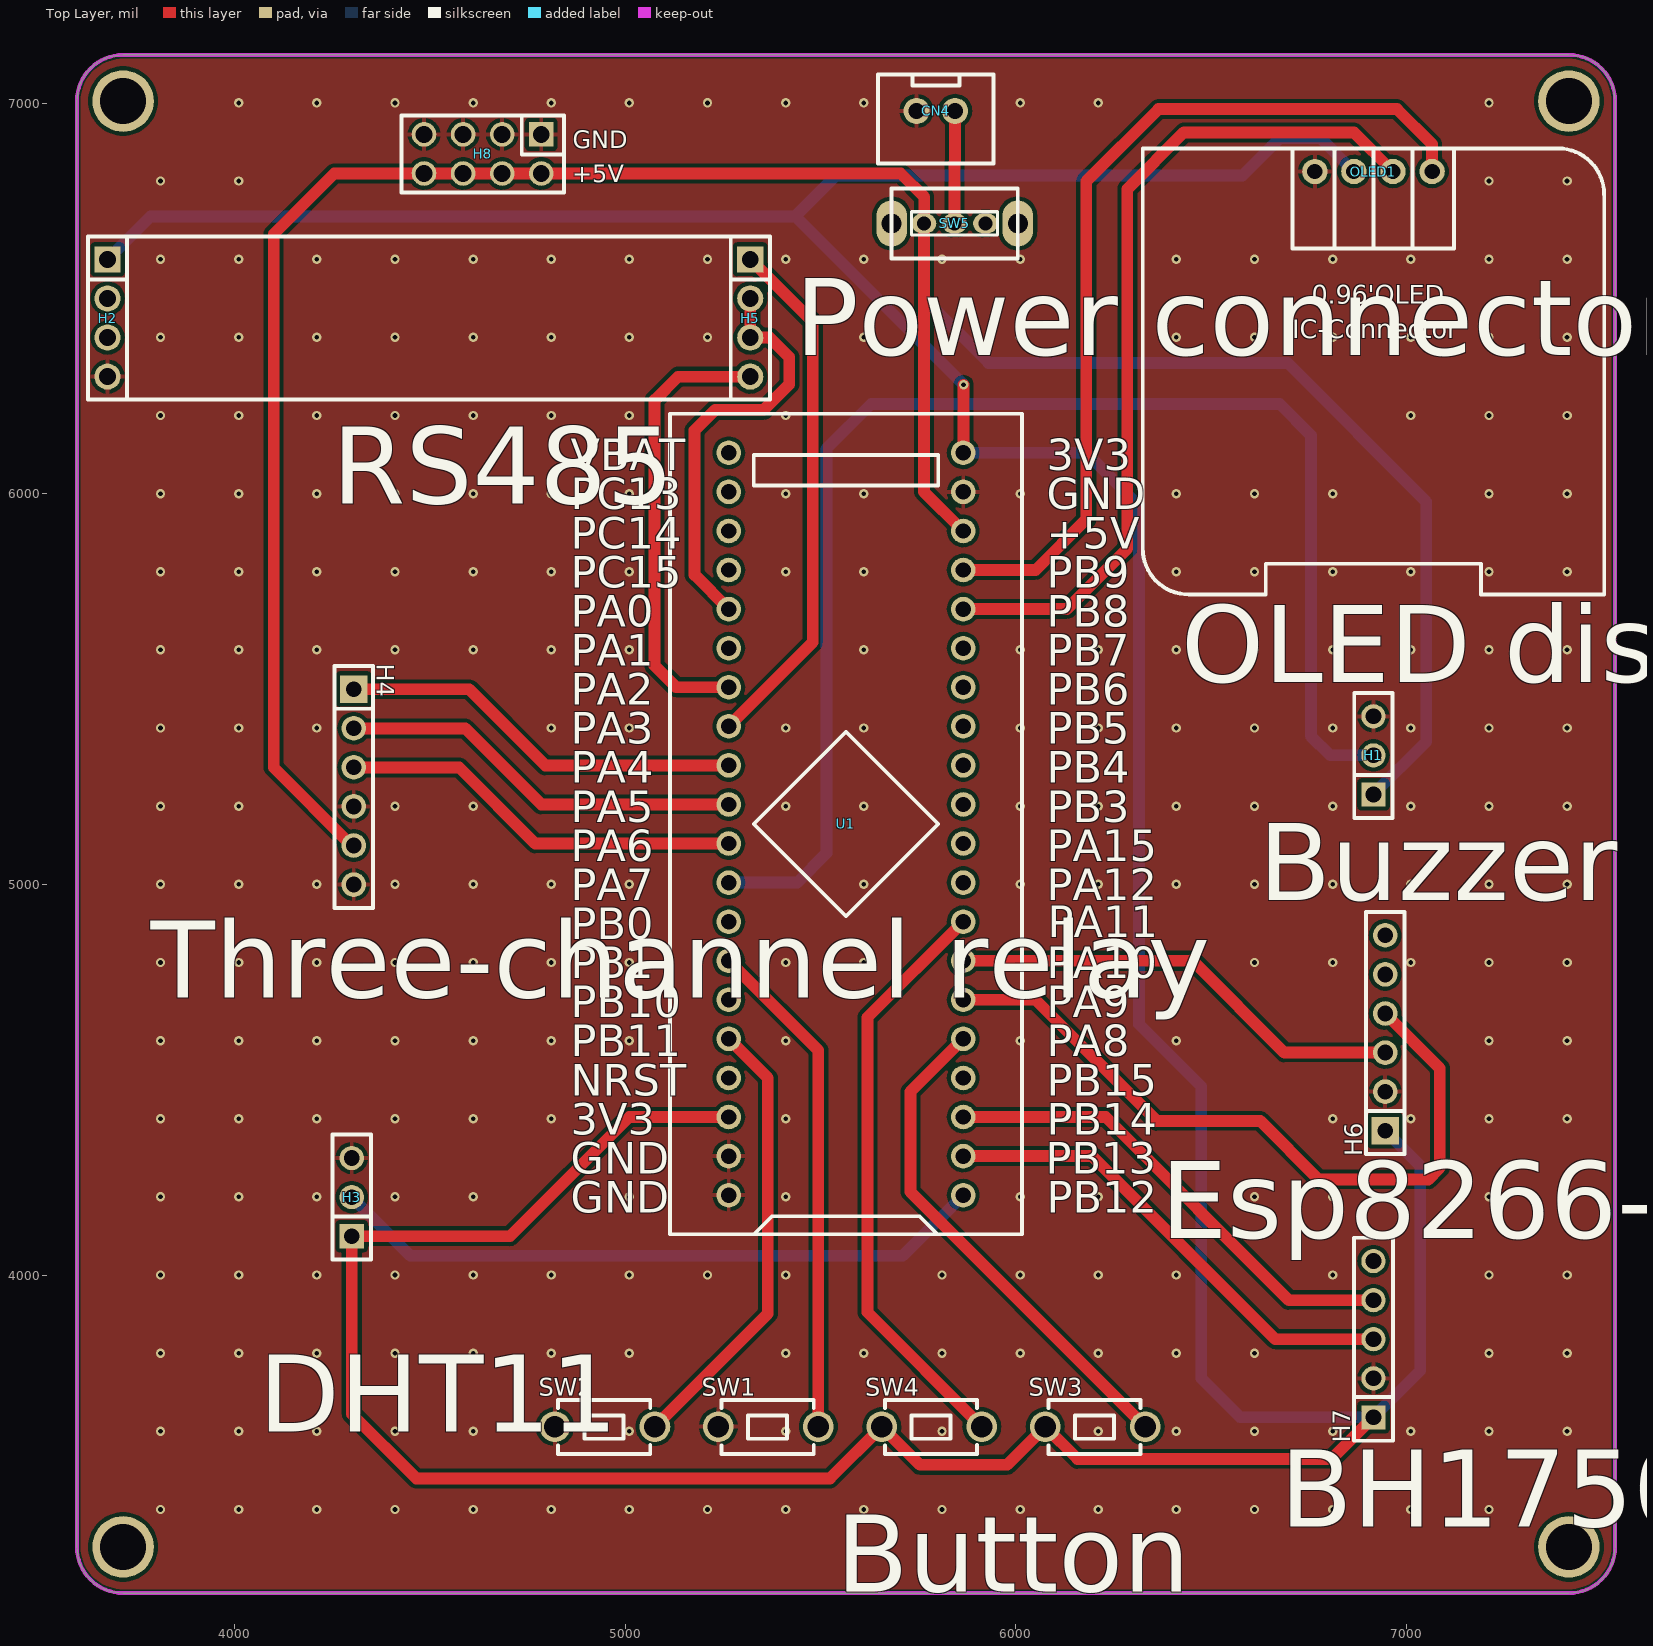
[diagram p0: Top Layer view]
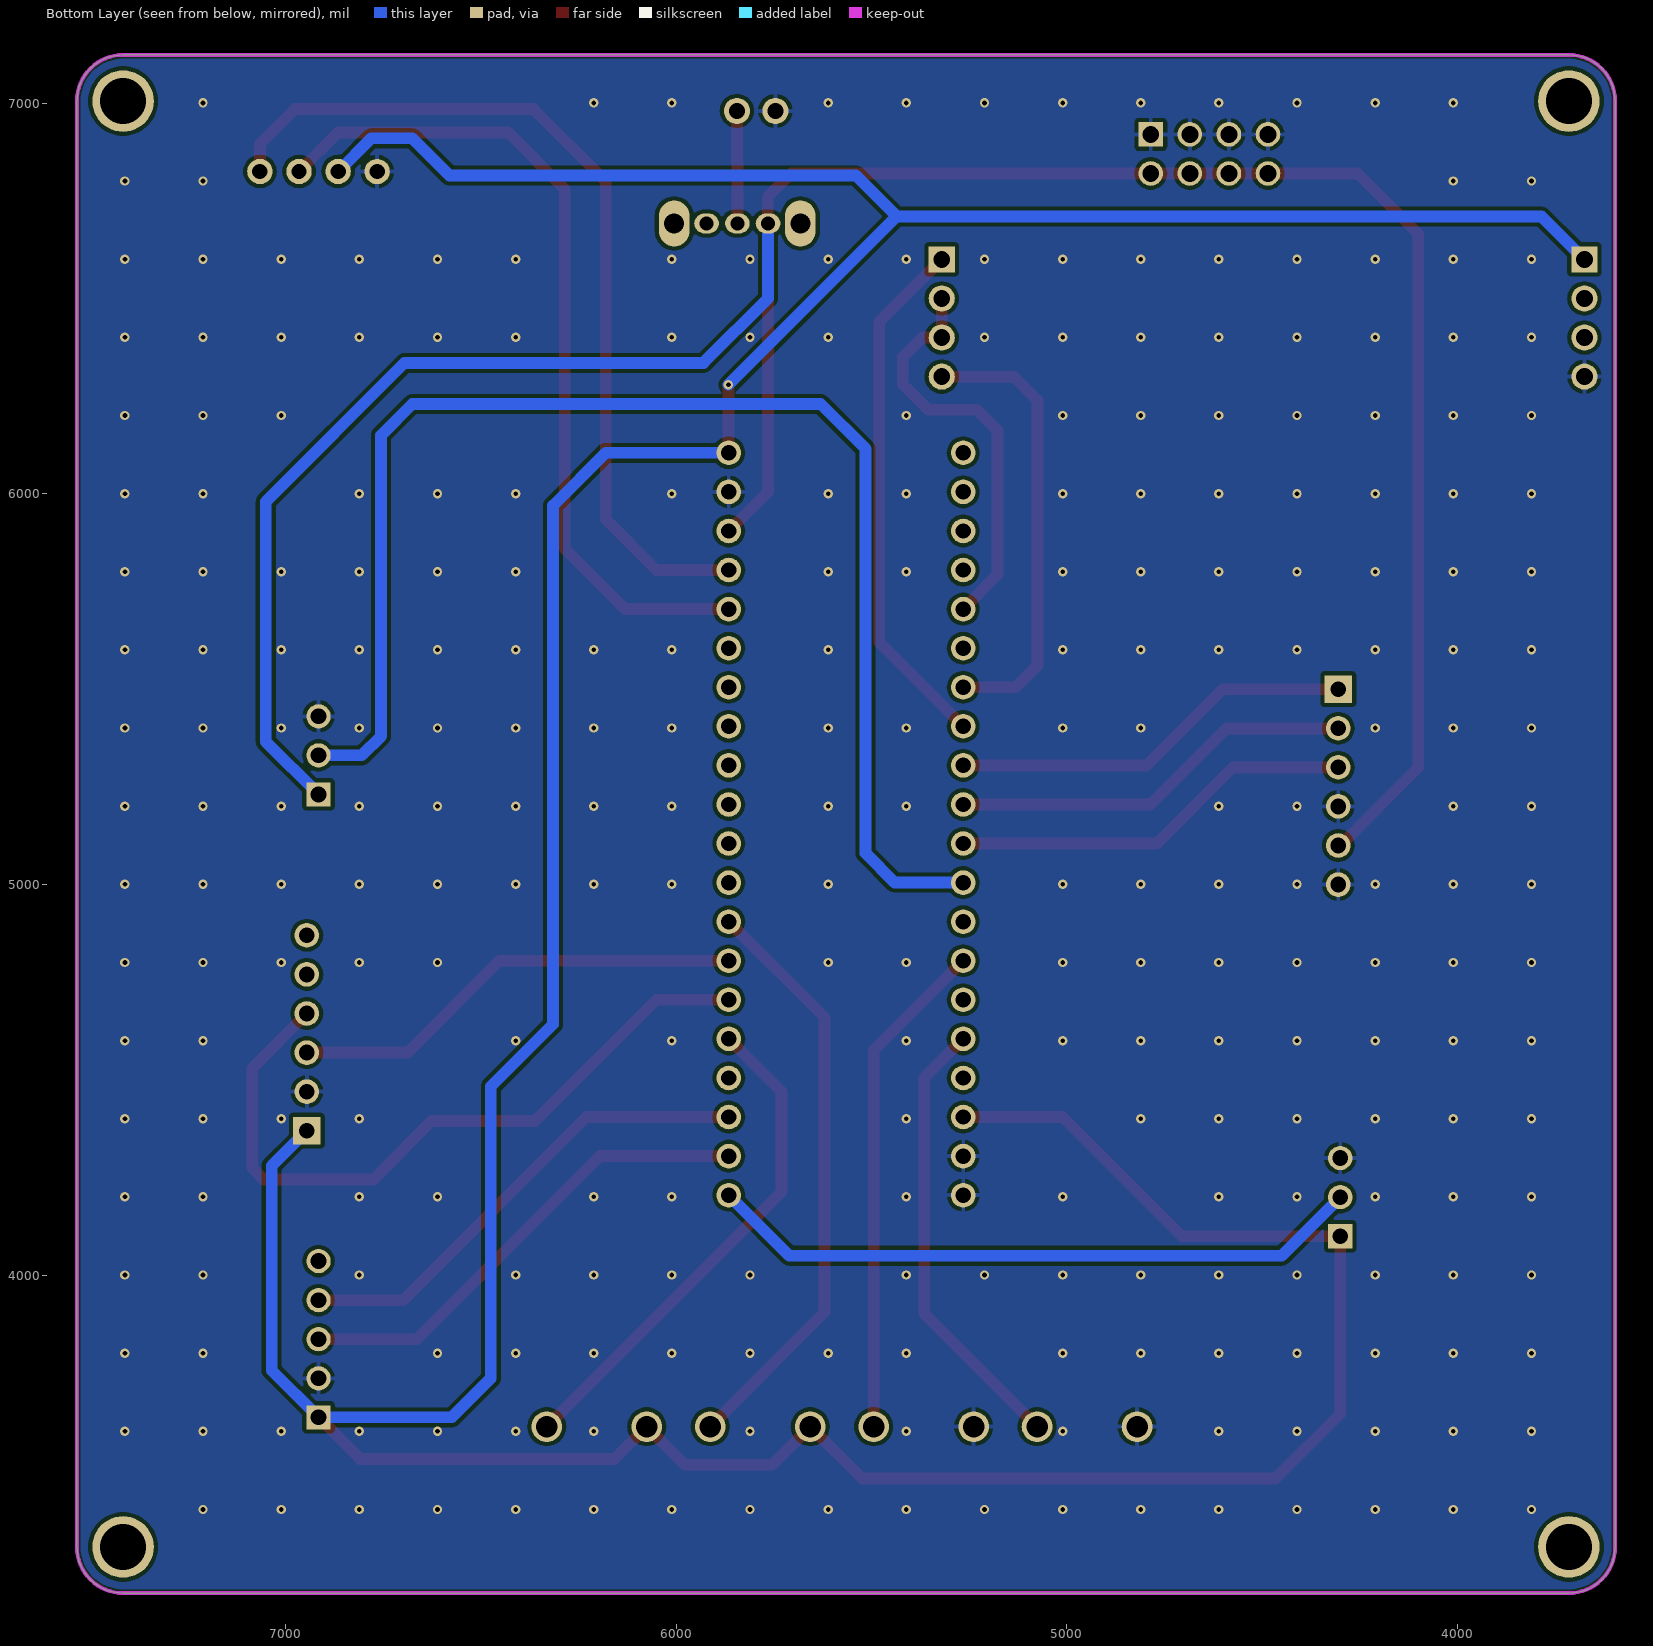
[diagram p1: Bottom Layer view, seen from below]
# Altium PCB MISC89004.pcbdoc
Units mil, origin at the board's own origin, x right, y up, seen from the top; angles counter-clockwise.
Board outline 3937.01 x 3937.01 mil, 2 copper layers (Top Layer, Bottom Layer), stack 62.206 mil thick; 16 components, 38 nets, 102 pads, 269 vias.

## Layer stack, top to bottom
Top Solder Mask Layer: solder mask 0.394, Dk 3.3
Top Layer: signal copper 1.379
Dielectric1: surface 59.449, FR4, Dk 4.5
Bottom Layer: signal copper 1.378
Bottom Solder Mask Layer: solder mask 0.394, Dk 3.3

## Board outline
3714.61,7123.5 ccw(c3714.61,7005.39) 3596.5,7005.39 3596.5,3304.61 ccw(c3714.61,3304.61) 3714.61,3186.5 7415.39,3186.5 ccw(c7415.39,3304.61) 7533.5,3304.61 7533.5,7005.39 ccw(c7415.39,7005.39) 7415.39,7123.5 3714.61,7123.5

## Design rules (kind name [scope] priority, off if disabled: settings)
BoardOutlineClearance copperThickness2oz_1 [All] p2 off: genericclearance=7.99 ignorepadtopadclearanceinfootprint=FALSE except(0: Arc-SplitContinuation Track-SplitContinuation SMDPad-SplitContinuation THPad-SplitContinuation Via-SplitContinuation Fill-SplitContinuation Region-SplitContinuation Poly-SplitContinuation Text-SplitContinuation Hole-SplitContinuation; 5.98: Arc-CutoutEdge Track-CutoutEdge SMDPad-CutoutEdge THPad-CutoutEdge Via-CutoutEdge Text-CutoutEdge; 6.9: Hole-OutlineEdge Hole-CutoutEdge; 10: Poly-OutlineEdge Poly-CutoutEdge; 11.81: Arc-OutlineEdge Track-OutlineEdge SMDPad-OutlineEdge THPad-OutlineEdge Via-OutlineEdge Fill-OutlineEdge Region-OutlineEdge Text-OutlineEdge Fill-CutoutEdge Region-CutoutEdge)
BoardOutlineClearance Plane_innerPlane_1 [All] p4 off: genericclearance=4.02 ignorepadtopadclearanceinfootprint=FALSE except(0: Arc-SplitContinuation Track-SplitContinuation SMDPad-SplitContinuation THPad-SplitContinuation Via-SplitContinuation Fill-SplitContinuation Region-SplitContinuation Poly-SplitContinuation Text-SplitContinuation Hole-SplitContinuation; 5.98: Arc-CutoutEdge Track-CutoutEdge SMDPad-CutoutEdge THPad-CutoutEdge Via-CutoutEdge Text-CutoutEdge; 6.9: Hole-OutlineEdge Hole-CutoutEdge; 10: Poly-OutlineEdge Poly-CutoutEdge; 11.81: Arc-OutlineEdge Track-OutlineEdge SMDPad-OutlineEdge THPad-OutlineEdge Via-OutlineEdge Fill-OutlineEdge Region-OutlineEdge Text-OutlineEdge Fill-CutoutEdge Region-CutoutEdge)
BoardOutlineClearance Copper_copperRegion_1 [All] p6 off: genericclearance=4.02 ignorepadtopadclearanceinfootprint=FALSE except(0: Arc-SplitContinuation Track-SplitContinuation SMDPad-SplitContinuation THPad-SplitContinuation Via-SplitContinuation Fill-SplitContinuation Region-SplitContinuation Poly-SplitContinuation Text-SplitContinuation Hole-SplitContinuation; 5.98: Arc-CutoutEdge Track-CutoutEdge SMDPad-CutoutEdge THPad-CutoutEdge Via-CutoutEdge Text-CutoutEdge; 6.9: Hole-OutlineEdge Hole-CutoutEdge; 10: Poly-OutlineEdge Poly-CutoutEdge; 11.81: Arc-OutlineEdge Track-OutlineEdge SMDPad-OutlineEdge THPad-OutlineEdge Via-OutlineEdge Fill-OutlineEdge Region-OutlineEdge Text-OutlineEdge Fill-CutoutEdge Region-CutoutEdge)
BoardOutlineClearance Copper_copperRegion_copperThickness1oz_1 [All] p8 off: genericclearance=4.02 ignorepadtopadclearanceinfootprint=FALSE except(0: Arc-SplitContinuation Track-SplitContinuation SMDPad-SplitContinuation THPad-SplitContinuation Via-SplitContinuation Fill-SplitContinuation Region-SplitContinuation Poly-SplitContinuation Text-SplitContinuation Hole-SplitContinuation; 5.98: Arc-CutoutEdge Track-CutoutEdge SMDPad-CutoutEdge THPad-CutoutEdge Via-CutoutEdge Text-CutoutEdge; 6.9: Hole-OutlineEdge Hole-CutoutEdge; 10: Poly-OutlineEdge Poly-CutoutEdge; 11.81: Arc-OutlineEdge Track-OutlineEdge SMDPad-OutlineEdge THPad-OutlineEdge Via-OutlineEdge Fill-OutlineEdge Region-OutlineEdge Text-OutlineEdge Fill-CutoutEdge Region-CutoutEdge)
BoardOutlineClearance Copper_copperRegion_Copper_copperRegion_1 [All] p10 off: genericclearance=4.02 ignorepadtopadclearanceinfootprint=FALSE except(0: Arc-SplitContinuation Track-SplitContinuation SMDPad-SplitContinuation THPad-SplitContinuation Via-SplitContinuation Fill-SplitContinuation Region-SplitContinuation Poly-SplitContinuation Text-SplitContinuation Hole-SplitContinuation; 5.98: Arc-CutoutEdge Track-CutoutEdge SMDPad-CutoutEdge THPad-CutoutEdge Via-CutoutEdge Text-CutoutEdge; 6.9: Hole-OutlineEdge Hole-CutoutEdge; 10: Poly-OutlineEdge Poly-CutoutEdge; 11.81: Arc-OutlineEdge Track-OutlineEdge SMDPad-OutlineEdge THPad-OutlineEdge Via-OutlineEdge Fill-OutlineEdge Region-OutlineEdge Text-OutlineEdge Fill-CutoutEdge Region-CutoutEdge)
BoardOutlineClearance copperThickness1oz_1 [All] p12: genericclearance=4.02 ignorepadtopadclearanceinfootprint=FALSE except(0: Arc-SplitContinuation Track-SplitContinuation SMDPad-SplitContinuation THPad-SplitContinuation Via-SplitContinuation Fill-SplitContinuation Region-SplitContinuation Poly-SplitContinuation Text-SplitContinuation Hole-SplitContinuation; 5.98: Arc-CutoutEdge Track-CutoutEdge SMDPad-CutoutEdge THPad-CutoutEdge Via-CutoutEdge Text-CutoutEdge; 6.9: Hole-OutlineEdge Hole-CutoutEdge; 10: Poly-OutlineEdge Poly-CutoutEdge; 11.81: Arc-OutlineEdge Track-OutlineEdge SMDPad-OutlineEdge THPad-OutlineEdge Via-OutlineEdge Fill-OutlineEdge Region-OutlineEdge Text-OutlineEdge Fill-CutoutEdge Region-CutoutEdge)
Clearance copperThickness2oz [All] p1 off: gap=7.99 ignorepadtopadclearanceinfootprint=FALSE except(5.98: SMDPad-Track SMDPad-SMDPad THPad-Track SMDPad-THPad THPad-THPad Track-Via SMDPad-Via THPad-Via Via-Via Fill-SMDPad Region-SMDPad Fill-THPad Region-THPad Fill-Via Region-Via Fill-Fill Fill-Region Region-Region Arc-Track Arc-SMDPad Arc-THPad Arc-Via Fill-Arc Region-Arc Arc-Arc Text-Track SMDPad-Text Text-THPad Text-Via Fill-Text Region-Text Arc-Text Text-Text; 6.9: Hole-Track Hole-SMDPad Hole-THPad Hole-Via Fill-Hole Region-Hole Hole-Arc Hole-Text; 10: Poly-Track Poly-SMDPad Poly-THPad Poly-Via Poly-Fill Poly-Region Poly-Poly Poly-Arc Poly-Text Poly-Hole; 11.81: Fill-Track Region-Track)
Clearance Plane_innerPlane [All] p3 off: gap=4.02 ignorepadtopadclearanceinfootprint=FALSE except(5.98: SMDPad-Track SMDPad-SMDPad THPad-Track SMDPad-THPad THPad-THPad Track-Via SMDPad-Via THPad-Via Via-Via Fill-SMDPad Region-SMDPad Fill-THPad Region-THPad Fill-Via Region-Via Fill-Fill Fill-Region Region-Region Arc-Track Arc-SMDPad Arc-THPad Arc-Via Fill-Arc Region-Arc Arc-Arc Text-Track SMDPad-Text Text-THPad Text-Via Fill-Text Region-Text Arc-Text Text-Text; 6.9: Hole-Track Hole-SMDPad Hole-THPad Hole-Via Fill-Hole Region-Hole Hole-Arc Hole-Text; 10: Poly-Track Poly-SMDPad Poly-THPad Poly-Via Poly-Fill Poly-Region Poly-Poly Poly-Arc Poly-Text Poly-Hole; 11.81: Fill-Track Region-Track)
Clearance Copper_copperRegion [All] p5 off: gap=4.02 ignorepadtopadclearanceinfootprint=FALSE except(5.98: SMDPad-Track SMDPad-SMDPad THPad-Track SMDPad-THPad THPad-THPad Track-Via SMDPad-Via THPad-Via Via-Via Fill-SMDPad Region-SMDPad Fill-THPad Region-THPad Fill-Via Region-Via Fill-Fill Fill-Region Region-Region Arc-Track Arc-SMDPad Arc-THPad Arc-Via Fill-Arc Region-Arc Arc-Arc Text-Track SMDPad-Text Text-THPad Text-Via Fill-Text Region-Text Arc-Text Text-Text; 6.9: Hole-Track Hole-SMDPad Hole-THPad Hole-Via Fill-Hole Region-Hole Hole-Arc Hole-Text; 10: Poly-Track Poly-SMDPad Poly-THPad Poly-Via Poly-Fill Poly-Region Poly-Poly Poly-Arc Poly-Text Poly-Hole; 11.81: Fill-Track Region-Track)
Clearance Copper_copperRegion_copperThickness1oz [All] p7 off: gap=4.02 ignorepadtopadclearanceinfootprint=FALSE except(5.98: SMDPad-Track SMDPad-SMDPad THPad-Track SMDPad-THPad THPad-THPad Track-Via SMDPad-Via THPad-Via Via-Via Fill-SMDPad Region-SMDPad Fill-THPad Region-THPad Fill-Via Region-Via Fill-Fill Fill-Region Region-Region Arc-Track Arc-SMDPad Arc-THPad Arc-Via Fill-Arc Region-Arc Arc-Arc Text-Track SMDPad-Text Text-THPad Text-Via Fill-Text Region-Text Arc-Text Text-Text; 6.9: Hole-Track Hole-SMDPad Hole-THPad Hole-Via Fill-Hole Region-Hole Hole-Arc Hole-Text; 10: Poly-Track Poly-SMDPad Poly-THPad Poly-Via Poly-Fill Poly-Region Poly-Poly Poly-Arc Poly-Text Poly-Hole; 11.81: Fill-Track Region-Track)
Clearance Copper_copperRegion_Copper_copperRegion [All] p9 off: gap=4.02 ignorepadtopadclearanceinfootprint=FALSE except(5.98: SMDPad-Track SMDPad-SMDPad THPad-Track SMDPad-THPad THPad-THPad Track-Via SMDPad-Via THPad-Via Via-Via Fill-SMDPad Region-SMDPad Fill-THPad Region-THPad Fill-Via Region-Via Fill-Fill Fill-Region Region-Region Arc-Track Arc-SMDPad Arc-THPad Arc-Via Fill-Arc Region-Arc Arc-Arc Text-Track SMDPad-Text Text-THPad Text-Via Fill-Text Region-Text Arc-Text Text-Text; 6.9: Hole-Track Hole-SMDPad Hole-THPad Hole-Via Fill-Hole Region-Hole Hole-Arc Hole-Text; 10: Poly-Track Poly-SMDPad Poly-THPad Poly-Via Poly-Fill Poly-Region Poly-Poly Poly-Arc Poly-Text Poly-Hole; 11.81: Fill-Track Region-Track)
Clearance copperThickness1oz [All] p11: gap=4.02 ignorepadtopadclearanceinfootprint=FALSE except(5.98: SMDPad-Track SMDPad-SMDPad THPad-Track SMDPad-THPad THPad-THPad Track-Via SMDPad-Via THPad-Via Via-Via Fill-SMDPad Region-SMDPad Fill-THPad Region-THPad Fill-Via Region-Via Fill-Fill Fill-Region Region-Region Arc-Track Arc-SMDPad Arc-THPad Arc-Via Fill-Arc Region-Arc Arc-Arc Text-Track SMDPad-Text Text-THPad Text-Via Fill-Text Region-Text Arc-Text Text-Text; 6.9: Hole-Track Hole-SMDPad Hole-THPad Hole-Via Fill-Hole Region-Hole Hole-Arc Hole-Text; 10: Poly-Track Poly-SMDPad Poly-THPad Poly-Via Poly-Fill Poly-Region Poly-Poly Poly-Arc Poly-Text Poly-Hole; 11.81: Fill-Track Region-Track)
DiffPairsRouting differentialPair [All] p1: maxlimit=6 minlimit=6 mostfreqgap=6 toplayer_minwidth=5 toplayer_prefwidth=10 toplayer_maxwidth=100 toplayer_mingap=6 toplayer_prefgap=6 toplayer_maxgap=6 bottomlayer_minwidth=5 bottomlayer_prefwidth=10 bottomlayer_maxwidth=100 bottomlayer_mingap=6 bottomlayer_prefgap=6 bottomlayer_maxgap=6 maxuncoupledlength=10
HoleToHoleClearance otherClearance [All] p1: gap=11.81 allowstackedmicrovias=TRUE
Length netLength [All] p1: minlimit=0 maxlimit=0
PasteMaskExpansion pasteMaskExpansion [All] p1: expansion=0
PlaneConnect innerPlane [All] p1: planeconnectstyle=Relief reliefexpansion=20 reliefentries=4 reliefconductorwidth=10 reliefairgap=10
PolygonConnect copperRegion_copperThickness1oz [All] p1 off: connectstyle=Relief reliefconductorwidth=10 reliefentries=4 polygonreliefangle="90 Angle" airgapwidth=10 via.connectstyle=Relief via.reliefconductorwidth=10 via.reliefentries=4 via.polygonreliefangle="90 Angle" via.airgapwidth=10
PolygonConnect copperRegion_Copper_copperRegion [All] p2 off: connectstyle=Relief reliefconductorwidth=10 reliefentries=4 polygonreliefangle="90 Angle" airgapwidth=10 via.connectstyle=Relief via.reliefconductorwidth=10 via.reliefentries=4 via.polygonreliefangle="90 Angle" via.airgapwidth=10
PolygonConnect copperRegion [All] p3: connectstyle=Relief reliefconductorwidth=10 reliefentries=4 polygonreliefangle="90 Angle" airgapwidth=10 via.connectstyle=Relief via.reliefconductorwidth=10 via.reliefentries=4 via.polygonreliefangle="90 Angle" via.airgapwidth=10
RoutingVias viaSize [All] p1: holewidth=12.01 width=24.02 viastyle="Through Hole" minholewidth=11.81 minwidth=19.68 maxholewidth=248.03 maxwidth=393.7
SolderMaskExpansion solderMaskExpansion [IsVia] p1: expansion=-1000 istentingtop=TRUE
SolderMaskExpansion solderMaskExpansion [All] p2: expansion=2 istentingtop=FALSE
Width copperThickness2oz_2 [All] p1 off: maxlimit=100 minlimit=8 preferedwidth=10
Width copperThickness1oz_2 [All] p2: maxlimit=100 minlimit=5 preferedwidth=10

## Components (designator, comment, footprint, x,y, rotation, side; value= is the part's Value field where it differs from the comment)
CN4 "XH2.54*2P_Straight" CONN-TH_2P-P2.50-XH2.54-2P 5795,6980 r0 top
H1 "" HDR-TH_3P-P2.54-V-F 6915,5330.66 r90 top
H2 "" HDR-TH_4P-P2.54-V-F 3675,6450 r270 top
H3 "" HDR-TH_3P-P2.54-V-F 4300,4199.99 r90 top
H4 "" HDR-TH_6P-P2.54-V-F 4305,5250 r270 top
H5 "" HDR-TH_4P-P2.54-V-F 5320,6450 r270 top
H6 "" HDR-TH_6P-P2.54-V-F 6945,4620 r90 top
H7 "" HDR-TH_5P-P2.54-V-F 6915,3836.3 r90 top
H8 "" HDR-TH_8P-P2.54-V-F-R2-C4-S2.54-1 4635,6870 r180 top
OLED1 "" 0.96OLED_4P 6915,6825 r0 top
SW1 "" Key_TH_3.5x6x4.3 5359.75,3612.61 r0 top
SW2 "" Key_TH_3.5x6x4.3 4941.42,3612.61 r0 top
SW3 "" Key_TH_3.5x6x4.3 6196.42,3612.61 r0 top
SW4 "" Key_TH_3.5x6x4.3 5778.08,3612.61 r0 top
SW5 "" 拨动开关 5837.9,6692.05 r0 top
U1 "STM32F103C8T6-Card" CONN-TH_L53.3-W22.9_STM32F103C8T6-CARD 5565,5155 r90 top

## Footprints (in the part's own frame and the unit in brackets; to place one, negate y for a bottom-side part, rotate by r counter-clockwise, add the part's x,y. Pads: shape width x height; smd on the part's side, far side on the other; paste and mask are expansions set on the pad)
0.96OLED_4P [mm]
  round 1.65 hole 1 copper offset 0,0: 1(-3.81,-0.001) 2(-1.27,0.002) 3(1.27,0.002) 4(3.81,0.002)
  silkscreen extent -15,-27.5 15,1.5
CONN-TH_2P-P2.50-XH2.54-2P [mm]
  round 1.7 hole 1.05 paste+0 mask+0.05: 1(1.25,0) 2(-1.25,0)
  silkscreen extent -3.75,-3.42 3.75,2.37
CONN-TH_L53.3-W22.9_STM32F103C8T6-CARD [mm]
  round 1.6 hole 1: 1(-24.13,-7.62) 2(-21.59,-7.62) 3(-19.05,-7.62) 4(-16.51,-7.62) 5(-13.97,-7.62) 6(-11.43,-7.62) 7(-8.89,-7.62) 8(-6.35,-7.62) 9(-3.81,-7.62) 10(-1.27,-7.62) 11(1.27,-7.62) 12(3.81,-7.62) 13(6.35,-7.62) 14(8.89,-7.62) 15(11.43,-7.62) 16(13.97,-7.62) 17(16.51,-7.62) 18(19.05,-7.62) 19(21.59,-7.62) 20(24.13,-7.62) 21(24.13,7.62) 22(21.59,7.62) 23(19.05,7.62) 24(16.51,7.62) 25(13.97,7.62) 26(11.43,7.62) 27(8.89,7.62) 28(6.35,7.62) 29(3.81,7.62) 30(1.27,7.62) 31(-1.27,7.62) 32(-3.81,7.62) 33(-6.35,7.62) 34(-8.89,7.62) 35(-11.43,7.62) 36(-13.97,7.62) 37(-16.51,7.62) 38(-19.05,7.62) 39(-21.59,7.62) 40(-24.13,7.62)
  silkscreen extent -26.67,-11.43 26.67,11.43
HDR-TH_3P-P2.54-V-F [mil]
  rect 62x62 hole 40.16: 1(-100,0)
  round 62 hole 40.16: 2(0,0) 3(100,0)
  silkscreen extent -160,-49 160,49
HDR-TH_4P-P2.54-V-F [mm]
  rect 1.7x1.7 hole 1.1: 1(-3.81,0)
  round 1.7 hole 1.1: 2(-1.27,0) 3(1.27,0) 4(3.81,0)
  silkscreen extent -5.29,-1.27 5.29,1.27
HDR-TH_5P-P2.54-V-F [mil]
  rect 62x62 hole 40.16: 1(-200,0)
  round 62 hole 40.16: 2(-100,0) 3(0,0) 4(100,0) 5(200,0)
  silkscreen extent -260,-50 260,50
HDR-TH_6P-P2.54-V-F [mm]
  rect 1.8x1.8 hole 1.02: 1(-6.35,0)
  round 1.6 hole 1.02: 2(-3.81,0) 3(-1.27,0) 4(1.27,0) 5(3.81,0) 6(6.35,0)
  silkscreen extent -7.87,-1.25 7.87,1.25
HDR-TH_8P-P2.54-V-F-R2-C4-S2.54-1 [mm]
  rect 1.6x1.6 hole 1.1: 1(-3.81,-1.27)
  round 1.6 hole 1.1: 2(-3.81,1.27) 3(-1.27,-1.27) 4(-1.27,1.27) 5(1.27,-1.27) 6(1.27,1.27) 7(3.81,-1.27) 8(3.81,1.27)
  silkscreen extent -5.28,-2.5 5.28,2.5
Key_TH_3.5x6x4.3 [mil]
  round 78.7 hole 55.1 paste+0 mask+2: A(-121.44,0) B(134.46,0)
  silkscreen extent -114,-70 123,68
拨动开关 [mil]
  oval 63x51.2 hole 35.4 paste+0 mask+2: 1(-73.4,0) 2(5,0) 3(84,0)
  oval 78.7x118.1 hole 51.2 paste+0 mask+2: 4(166.7,0) 5(-156.1,0)
  silkscreen extent -156,-90 167,90

## Free pads (board coordinates)
  round 157.48 hole 118.11: 1(3714.61,7005.39) 1(3714.61,3304.61) 1(7415.39,7005.39) 1(7415.39,3304.61)

## Via types
v1: diameter 24.02, hole 12, Top Layer to Bottom Layer, 269 vias

## Nets (pads, with @x,y where several pads share a name; then routed paths per layer and width w, separated by ;. In a path a pad name is that pad's centre, name@x,y a point inside that pad or via, vN(x,y) a via of type N, cw(c..) or ccw(c..) an arc to the next point about the centre after c; other vN are vias at no path point)
$1N17118: CN4.1 SW5.2 | length 288.5
  Top Layer w30: SW5.2 5842.9,6847.1 5844.22,6848.41 CN4.1
+5V: H1.1 H4.5 H8.2 H8.4 H8.6 H8.8 SW5.1 U1.18 | length 6797.1
  Top Layer w30: H4.5@4300,5099.56 4100,5299.56 4100,6665 4255,6820 H8.8 H8.6 H8.4 H8.2 5705,6820 5765,6760 5765,6692.55 SW5.1 5764.5,6005.5 U1.18
  Bottom Layer w30: SW5.1 5764.5,6500.5 5930,6335 6695,6335 7050,5980 7050,5365.66 H1.1
D1: H5.4 U1.27 | length 1162.6
  Top Layer w30: U1.27 5130,5505 5075,5560 5075,6240 5135,6300 H5.4
DE: H5.2 H5.3 U1.25 | length 1075.6
  Top Layer w30: U1.25 5177.5,5792.5 5177.5,6162.5 5230,6215 5355,6215 5420,6280 5420,6350 5370,6400 H5.3 H5.2
GND: CN4.2 H1.3 H2.4 H3.3 H4.4 H4.6 H6.2 H7.2 H8.1 H8.3 H8.5 H8.7 OLED1.1 SW1.A SW2.A U1.19 U1.39 U1.40
  other v1: 3810.6,3400.6 4010.6,3400.6 4210.6,3400.6 4410.6,3400.6 4610.6,3400.6 4810.6,3400.6 5010.6,3400.6 5210.6,3400.6 5410.6,3400.6 5610.6,3400.6 5810.6,3400.6 6010.6,3400.6 6210.6,3400.6 6410.6,3400.6 6610.6,3400.6 6810.6,3400.6 7010.6,3400.6 7210.6,3400.6 3810.6,3600.6 4010.6,3600.6 4210.6,3600.6 4410.6,3600.6 4610.6,3600.6 5010.6,3600.6 5410.6,3600.6 5810.6,3600.6 6210.6,3600.6 6410.6,3600.6 6610.6,3600.6 6810.6,3600.6 7010.6,3600.6 7210.6,3600.6 7410.6,3600.6 3810.6,3800.6 4010.6,3800.6 4210.6,3800.6 4410.6,3800.6 4610.6,3800.6 4810.6,3800.6 5010.6,3800.6 5410.6,3800.6 5610.6,3800.6 5810.6,3800.6 6010.6,3800.6 6210.6,3800.6 6410.6,3800.6 6610.6,3800.6 7210.6,3800.6 7410.6,3800.6 3810.6,4000.6 4010.6,4000.6 4210.6,4000.6 4410.6,4000.6 4610.6,4000.6 4810.6,4000.6 5010.6,4000.6 5210.6,4000.6 5410.6,4000.6 5810.6,4000.6 6010.6,4000.6 6210.6,4000.6 6410.6,4000.6 6810.6,4000.6 7210.6,4000.6 7410.6,4000.6 3810.6,4200.6 4010.6,4200.6 4210.6,4200.6 4410.6,4200.6 4610.6,4200.6 5010.6,4200.6 5410.6,4200.6 6010.6,4200.6 6210.6,4200.6 6610.6,4200.6 6810.6,4200.6 7210.6,4200.6 7410.6,4200.6 3810.6,4400.6 4010.6,4400.6 4210.6,4400.6 4410.6,4400.6 4610.6,4400.6 4810.6,4400.6 5410.6,4400.6 6810.6,4400.6 7010.6,4400.6 7210.6,4400.6 7410.6,4400.6 3810.6,4600.6 4010.6,4600.6 4210.6,4600.6 4410.6,4600.6 4610.6,4600.6 4810.6,4600.6 5010.6,4600.6 5410.6,4600.6 6010.6,4600.6 6410.6,4600.6 7210.6,4600.6 7410.6,4600.6 3810.6,4800.6 4010.6,4800.6 4210.6,4800.6 4410.6,4800.6 4610.6,4800.6 4810.6,4800.6 5010.6,4800.6 5410.6,4800.6 5610.6,4800.6 6610.6,4800.6 6810.6,4800.6 7010.6,4800.6 7210.6,4800.6 7410.6,4800.6 3810.6,5000.6 4010.6,5000.6 4210.6,5000.6 4410.6,5000.6 4610.6,5000.6 4810.6,5000.6 5010.6,5000.6 5610.6,5000.6 6010.6,5000.6 6210.6,5000.6 6410.6,5000.6 6610.6,5000.6 6810.6,5000.6 7010.6,5000.6 7210.6,5000.6 7410.6,5000.6 3810.6,5200.6 4010.6,5200.6 4410.6,5200.6 4610.6,5200.6 5410.6,5200.6 5610.6,5200.6 6010.6,5200.6 6210.6,5200.6 6410.6,5200.6 6610.6,5200.6 6810.6,5200.6 7010.6,5200.6 7210.6,5200.6 7410.6,5200.6 3810.6,5400.6 4010.6,5400.6 4210.6,5400.6 4810.6,5400.6 5010.6,5400.6 5410.6,5400.6 5610.6,5400.6 6010.6,5400.6 6210.6,5400.6 6410.6,5400.6 6610.6,5400.6 6810.6,5400.6 7010.6,5400.6 7210.6,5400.6 7410.6,5400.6 3810.6,5600.6 4010.6,5600.6 4210.6,5600.6 4410.6,5600.6 4610.6,5600.6 4810.6,5600.6 5010.6,5600.6 5610.6,5600.6 6010.6,5600.6 6210.6,5600.6 6410.6,5600.6 6610.6,5600.6 6810.6,5600.6 7010.6,5600.6 7210.6,5600.6 7410.6,5600.6 3810.6,5800.6 4010.6,5800.6 4210.6,5800.6 4410.6,5800.6 4610.6,5800.6 4810.6,5800.6 5010.6,5800.6 5410.6,5800.6 5610.6,5800.6 6410.6,5800.6 6610.6,5800.6 6810.6,5800.6 7010.6,5800.6 7210.6,5800.6 7410.6,5800.6 3810.6,6000.6 4010.6,6000.6 4210.6,6000.6 4410.6,6000.6 4610.6,6000.6 4810.6,6000.6 5010.6,6000.6 5410.6,6000.6 5610.6,6000.6 6010.6,6000.6 6410.6,6000.6 6610.6,6000.6 6810.6,6000.6 7210.6,6000.6 7410.6,6000.6 3810.6,6200.6 4010.6,6200.6 4210.6,6200.6 4410.6,6200.6 4610.6,6200.6 4810.6,6200.6 5010.6,6200.6 5410.6,6200.6 7010.6,6200.6 7210.6,6200.6 7410.6,6200.6 3810.6,6400.6 4010.6,6400.6 4210.6,6400.6 4410.6,6400.6 4610.6,6400.6 4810.6,6400.6 5010.6,6400.6 5210.6,6400.6 5610.6,6400.6 5810.6,6400.6 6010.6,6400.6 6410.6,6400.6 6610.6,6400.6 6810.6,6400.6 7010.6,6400.6 7210.6,6400.6 7410.6,6400.6 3810.6,6600.6 4010.6,6600.6 4210.6,6600.6 4410.6,6600.6 4610.6,6600.6 4810.6,6600.6 5010.6,6600.6 5210.6,6600.6 5410.6,6600.6 5610.6,6600.6 5810.6,6600.6 6010.6,6600.6 6410.6,6600.6 6610.6,6600.6 6810.6,6600.6 7010.6,6600.6 7210.6,6600.6 7410.6,6600.6 3810.6,6800.6 4010.6,6800.6 7210.6,6800.6 7410.6,6800.6 4010.6,7000.6 4210.6,7000.6 4410.6,7000.6 4610.6,7000.6 4810.6,7000.6 5010.6,7000.6 5210.6,7000.6 5410.6,7000.6 5610.6,7000.6 6010.6,7000.6 6210.6,7000.6 7210.6,7000.6
NRST: U1.37
PA1: U1.26
PA3: H5.1 U1.28 | length 1350.3
  Top Layer w30: U1.28 5480,5620 5480,6440 H5.1
PA4: H4.1 U1.29 | length 1045.6
  Top Layer w30: H4.1@4300,5499.56 4600.44,5499.56 4795,5305 U1.29
PA5: H4.2 U1.30 | length 1045.6
  Top Layer w30: H4.2@4300,5399.56 4590.44,5399.56 4785,5205 U1.30
PA6: H4.3 U1.31 | length 1045.6
  Top Layer w30: H4.3@4300,5299.56 4575.44,5299.56 4770,5105 U1.31
PA7: H1.2 U1.32 | length 3587.3
  Bottom Layer w30: U1.32 5440,5005 5515,5080 5515,6115 5630,6230 6675,6230 6755,6150 6755,5380 6804.34,5330.66 H1.2
PA8: SW3.B U1.5 | length 1297.2
  Top Layer w30: U1.5 5730,4470 5730,4213.49 SW3.B
PA9: H6.4 U1.6 | length 1876
  Top Layer w30: U1.6 6050,4705 6360,4395 6625,4395 6775,4245 7055,4245 7085,4275 7085,4530 H6.4
PA10: H6.3 U1.7 | length 1177.3
  Top Layer w30: U1.7 6452.17,4805 6687.18,4570 H6.3
PA11: SW4.B U1.8 | length 1515
  Top Layer w30: U1.8 5620,4660 5620,3905.16 SW4.B
PA12: U1.9
PA15: U1.10
PB0: U1.33
PB1: SW1.B U1.34 | length 1287.3
  Top Layer w30: U1.34 5494.21,4575.79 SW1.B
PB3: U1.11
PB4: U1.12
PB5: U1.13
PB6: U1.14
PB7: U1.15
PB8: OLED1.3 U1.16 | length 2185.7
  Top Layer w30: U1.16 6130,5705 6285,5860 6285,6780 6430,6925 6865.05,6925 OLED1.3@6965,6825.05
PB9: OLED1.4 U1.17 | length 2302.7
  Top Layer w30: U1.17 6050,5805 6180,5935 6180,6800 6365,6985 6975,6985 7065,6895 OLED1.4@7065,6825.05
PB10: U1.35
PB11: SW2.B U1.36 | length 1153.6
  Top Layer w30: SW2.B 5365,3901.74 5365,4505 U1.36
PB12: H3.2 U1.1 | length 1691.3
  Bottom Layer w30: H3.2 4449.99,4050 5710,4050 U1.1
PB13: H7.3 U1.2 | length 1244.1
  Top Layer w30: U1.2 6195,4305 6663.7,3836.3 H7.3
PB14: H7.4 U1.3 | length 1244.1
  Top Layer w30: U1.3 6230,4405 6698.7,3936.3 H7.4
PB15: U1.4
PC13: U1.22
PC14: U1.23
PC15: U1.24
VBAT: U1.21
VCC: H2.1 H3.1 H6.1 H7.1 OLED1.2 SW3.A SW4.A U1.20 U1.38 | length 12689.9
  Top Layer w30: U1.38 5010,4405 4704.99,4099.99 H3.1 4300,3645 4465,3480 5524.03,3480 SW4.A 5754.26,3515 5977.36,3515 SW3.A 6157.59,3530 6808.7,3530 H7.1 ; U1.20 5865.9,6105.9 v1(5865.9,6279.1)
  Bottom Layer w30: H2.1 3785,6710 5435,6710 ; U1.20 6180,6105 6315,5970 6315,4642.18 6474,4483.18 6474,3736 6573.7,3636.3 H7.1 7035,3756.3 7035,4280 H6.1 ; v1(5865.9,6279.1) 5435,6710 ; OLED1.2@6865,6825.05 6780.05,6910 6675,6910 6580,6815 5540,6815 5435,6710
pads on no net: H2.2 H2.3 H6.5 H6.6 H7.5 SW5.3 SW5.4 SW5.5

## Polygon pours and split planes (outlines as drawn)
GND on Bottom Layer (solid, remove dead copper, pour order 2): 3525,7245 3525,3080 7700,3080 7700,7245
GND on Top Layer (solid, remove dead copper, pour order 2): 3000,7415 3000,3000 7930,3000 7930,7415

## Keep-outs
Board Outline Layer:
  the board outline again, w10

## Silkscreen, mask and mechanical layers (free items; w line width, h text height)
Top Silkscreen Layer:
  lines w10: 3625,6241.73 3625,6658.27 5370,6658.27 5370,6241.73 3625,6241.73
  text "GND" at 4865,6885 h45
  text "+5V" at 4864.49,6797.5 h45
  text "Power connector" at 5435,6355 h196.85
  text "VBAT" at 4860.95,6060 h80
  text "3V3" at 6079.16,6060 h80
  text "RS485" at 4250,5975 h196.85
  text "PC13" at 4860.95,5960 h80
  text "GND" at 6079.16,5960 h80
  text "PC14" at 4860.95,5860 h80
  text "+5V" at 6079.16,5860 h80
  text "PC15" at 4860.95,5760 h80
  text "PB9" at 6079.16,5760 h80
  text "PA0" at 4860.95,5660 h80
  text "PB8" at 6079.16,5660 h80
  text "PA1" at 4860.95,5560 h80
  text "PB7" at 6079.16,5560 h80
  text "OLED display" at 6423.02,5518 h196.85
  text "PA2" at 4860.95,5460 h80
  text "PB6" at 6079.16,5460 h80
  text "PA3" at 4860.95,5360 h80
  text "PB5" at 6079.16,5360 h80
  text "PA4" at 4860.95,5260 h80
  text "PB4" at 6079.16,5260 h80
  text "PA5" at 4860.95,5160 h80
  text "PB3" at 6079.16,5160 h80
  text "PA6" at 4860.95,5060 h80
  text "PA15" at 6079.16,5060 h80
  text "PA7" at 4860.95,4960 h80
  text "PA12" at 6079.16,4960 h80
  text "Buzzer" at 6621.81,4960.19 h196.85
  text "PA11" at 6080.95,4865 h80
  text "PB0" at 4860.95,4860 h80
  text "PB1" at 4860.95,4760 h80
  text "PA10" at 6079.16,4760 h80
  text "Three-channel relay" at 3785,4710 h196.85
  text "PB10" at 4860.95,4660 h80
  text "PA9" at 6079.16,4660 h80
  text "PB11" at 4860.95,4560 h80
  text "PA8" at 6079.16,4560 h80
  text "NRST" at 4860.95,4460 h80
  text "PB15" at 6079.16,4460 h80
  text "3V3" at 4860.95,4360 h80
  text "PB14" at 6079.16,4360 h80
  text "GND" at 4860.95,4260 h80
  text "PB13" at 6075.95,4260 h80
  text "GND" at 4860.95,4160 h80
  text "PB12" at 6079.16,4160 h80
  text "Esp8266-01s" at 6370,4095 h196.85
  text "DHT11" at 4061.39,3600 h196.85
  text "BH1750" at 6676.39,3356.57 h196.85
  text "Button" at 5540,3190 h196.85